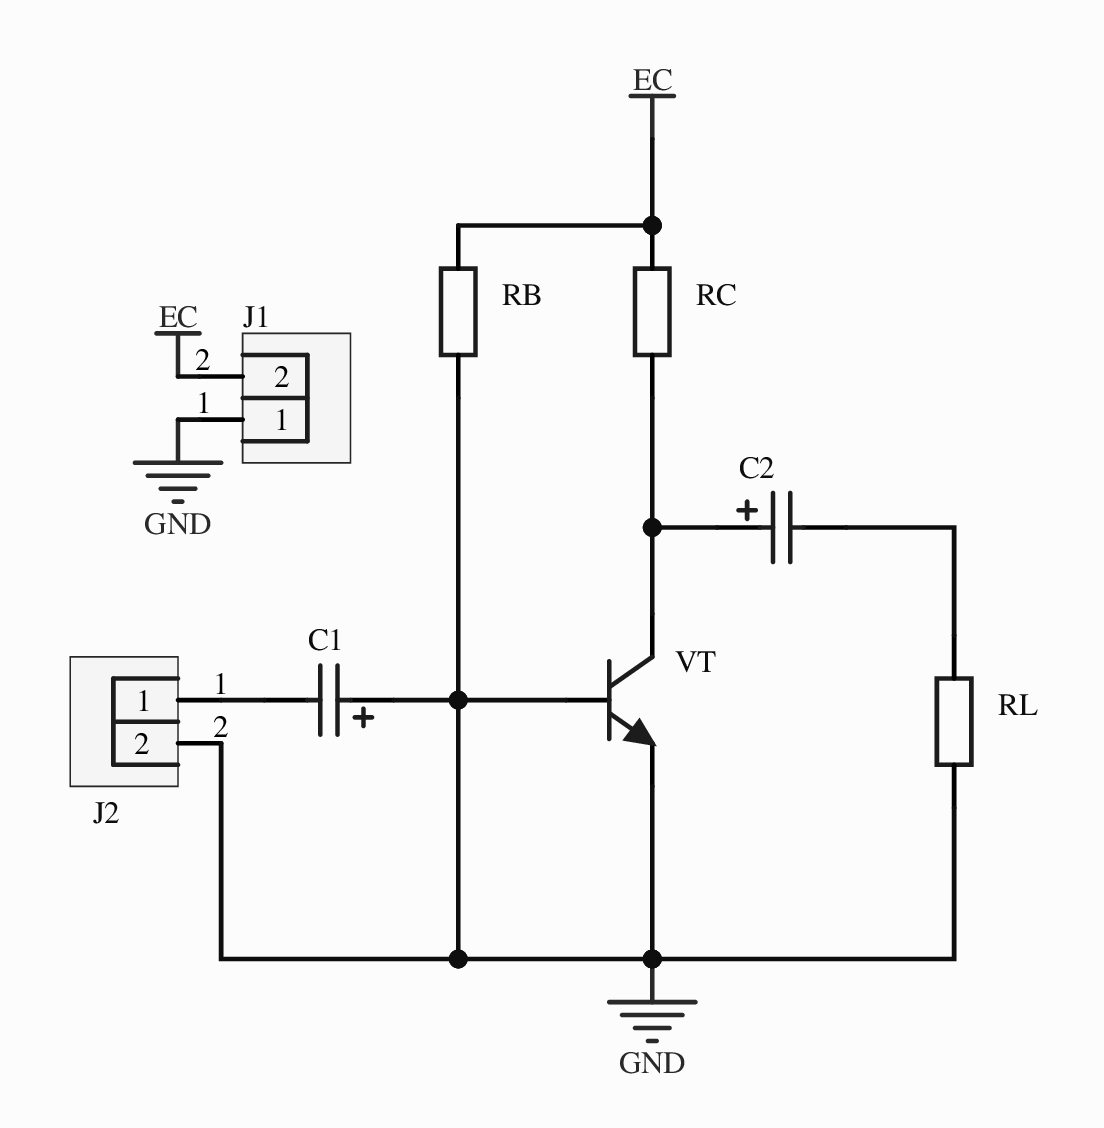
[diagram p0: MISC51134-3.schdoc]
# Altium project MISC51134-2.PrjPcb
1 sheet, 8 parts. Net scope: global (net labels, ports and power ports of the same name join across sheets).
Board file: MISC51134.pcbdoc

## Sheet MISC51134-3.schdoc
size 210 x 148 mm; Version: V1.0; @Project Name: MISC51134; @Update Date: 2026-10-07; @Create Date: 2026-10-07; @Board Name: MISC51134; @Create Time: 12:44:54; @Page Count: 1; @Page No: 1; @Schematic Name: MISC51134; @Update Time: 12:44:54; Size: A4

### Parts
C1  100pF  [C_Ele_SMD_3x5.4mm]  (value not drawn)
C2  100pF  [C_Ele_SMD_3x5.4mm]  (value not drawn)
J1  (no value)  [HDR-TH_2P-P2.54-V-M-1]
J2  (no value)  [HDR-TH_2P-P2.54-V-M-1]
RB  5.1K  [R0603]  (value not drawn)
RC  1K  [R0603]  (value not drawn)
RL  1K  [R0603]  (value not drawn)
VT  (no value)  [S8050_SOT-23]

### Nets
EC: J1.2 RB.2 RC.2
GND: C1.1 J1.1 J2.2 RB.1 RL.1 VT.1 VT.2
NetC1_2: C1.2 J2.1
NetC2_1: C2.1 RC.1 VT.3
NetC2_2: C2.2 RL.2

### Library data of the parts
C1 C2 = C_Ele_SMD_3x5.4mm: Symbol: CAP_OLD; AddInBom: yes; ModelId: 0132c3d3fdbf4fd987f710a97e7a5b5d0819f05c4eef4c71ace90d822a990e87; ModelName: CAP-SMD_BD3.0-L3.3-W3.3-H5.3; ModelTransform: 129.9,149.58,209.06,-90,0,0,0,0,0; Device: C_Ele_SMD_3x5.4mm; Value: 100pF; FootprintName: C_Ele_SMD_3x5.4mm; Supplier Footprint: SMD,3x5.4mm; ConvertToPcb: yes
J1 = HDR-M_2.54_1x2P: Symbol: 210S-1*2P L=11.6MMGold-plated black; 3D Model: 79b2e9f2d70a4d68a1b7098f27c6d4c50819f05c4eef4c71ace90d822a990e87; 3D Model Transform: 200,100,0,0,0,0,0,0,-118.11; ConvertToPcb: yes; ModelName: HDR-M-2.54_1x2; Device: HDR-M_2.54_1x2P; Supplier Part: C124375; Supplier Footprint: 插件; FootprintName: HDR-TH_2P-P2.54-V-M-1; AddInBom: yes
J2 = HDR-M_2.54_1x2P: Symbol: 210S-1*2P L=11.6MMGold-plated black; ConvertToPcb: yes; ModelId: 79b2e9f2d70a4d68a1b7098f27c6d4c50819f05c4eef4c71ace90d822a990e87; ModelName: HDR-M-2.54_1x2; ModelTransform: 200,100,0,0,0,0,0,0,-118.11; Device: HDR-M_2.54_1x2P; FootprintName: HDR-TH_2P-P2.54-V-M-1; AddInBom: yes; SupplierPart: C124375; Supplier Footprint: 插件
RB RC RL = Res_0603: Symbol: 电阻; 3D Model: fc143cca1e79419f9cd78b61e9279f080819f05c4eef4c71ace90d822a990e87; 3D Model Transform: 31.8897,63.7794,0,90,0,0,0,0,0; ConvertToPcb: yes; Device: Res_0603; Supplier Footprint: 0603; FootprintName: R0603; AddInBom: yes; ModelName: R0603
  RB: Value: 5.1K
  RC RL: Value: 1K
VT = S8050_SOT_NPN: Symbol: NPN; ConvertToPcb: yes; ModelId: c62791f0466c4ae2a892c056b845b0ca0819f05c4eef4c71ace90d822a990e87; ModelName: SOT-23-3P_L2.9-W1.3-H1.0-LS2.4-P0.95; ModelTransform: 98.6,114.12,41.29,180,0,0,0,0,-3; Device: S8050_SOT_NPN; FootprintName: S8050_SOT-23; AddInBom: yes; Supplier Footprint: SOT-23